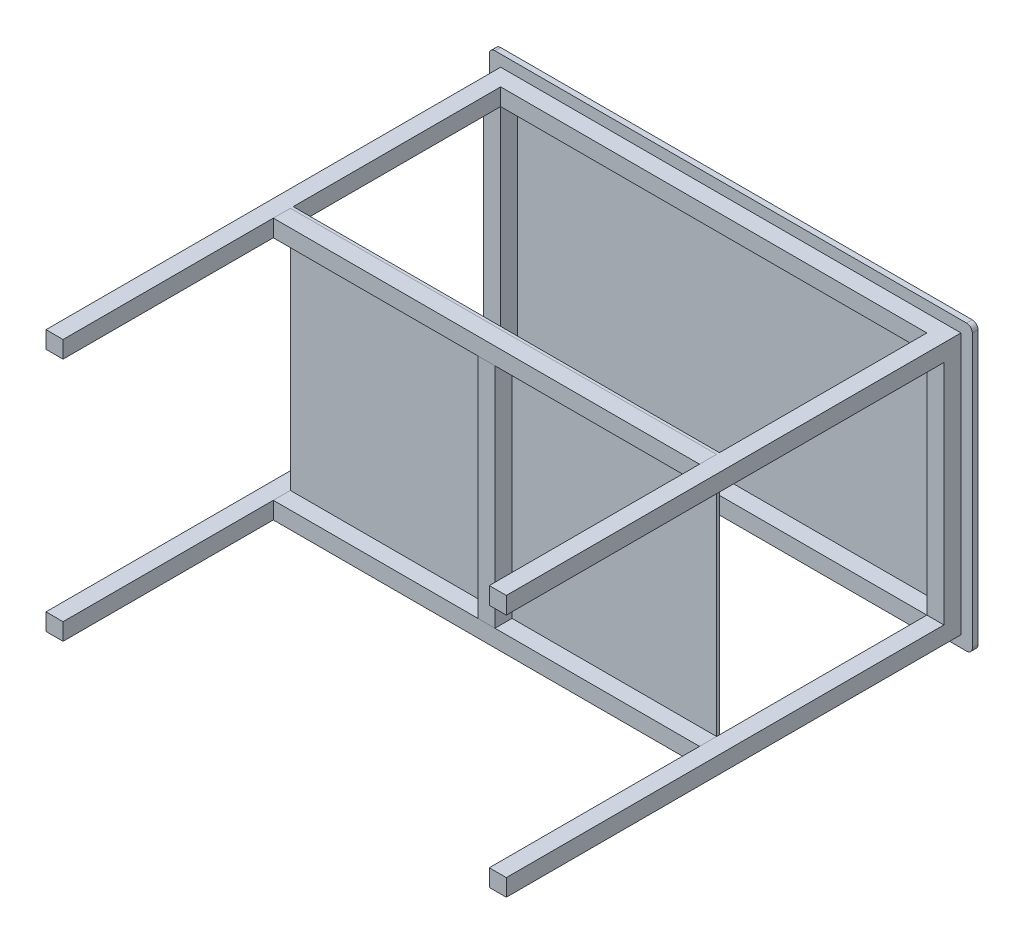
SolidWorks part; units mm, degrees
ref_plane "前视基准面" through (0, 0, 0) normal (0, 0, 1) x (1, 0, 0)
ref_plane "上视基准面" through (0, 0, 0) normal (0, 1, 0) x (1, 0, 0)
ref_plane "右视基准面" through (0, 0, 0) normal (1, 0, 0) x (0, 0, -1)
sketch "草图1" plane through (0, 0, 0) normal (0, 0, 1) x (1, 0, 0)
  line L1 (-425, 250) -> (425, 250)
  line L2 (-425, 250) -> (-425, -250)
  line L3 (-425, -250) -> (425, -250)
  line L4 (425, 250) -> (425, -250)
  line L5 (-425, 250) -> (425, -250) construction
  line L6 (-425, -250) -> (425, 250) construction
  point P0 (0, 0)
  dimension "D1" = 850
  dimension "D2" = 500
extrude "凸台-拉伸1" add sketch "草图1" along normal blind 10
sketch "草图2" plane through (0, 0, 10) normal (0, 0, 1) x (1, 0, 0)
  line L0 (425, 250) -> (-425, 250) construction
  line L1 (-405, 230) -> (405, 230)
  line L2 (-405, 230) -> (-405, -230)
  line L3 (-405, -230) -> (405, -230)
  line L4 (405, 230) -> (405, -230)
  line L5 (-405, 230) -> (405, -230) construction
  line L6 (-405, -230) -> (405, 230) construction
  line L7 (-425, 250) -> (-425, -250) construction
  line L8 (-375, 200) -> (-375, -200)
  line L9 (-375, -200) -> (375, -200)
  line L10 (375, 200) -> (375, -200)
  line L11 (-375, 200) -> (375, 200)
  point P0 (0, 0)
  dimension "D1" = 20
  dimension "D2" = 20
  dimension "D3" = 30
extrude "凸台-拉伸2" add sketch "草图2" along normal blind 30 separate body
sketch "草图3" plane through (0, 0, 40) normal (0, 0, 1) x (1, 0, 0)
  line L1 (-405, 230) -> (-375, 230)
  line L2 (-405, 230) -> (-405, 200)
  line L3 (-405, 200) -> (-375, 200)
  line L4 (-375, 230) -> (-375, 200)
  line L5 (375, -200) -> (405, -200)
  line L6 (375, -200) -> (375, -230)
  line L7 (375, -230) -> (405, -230)
  line L8 (405, -200) -> (405, -230)
  line L9 (405, 230) -> (375, 230)
  line L10 (405, 230) -> (405, 200)
  line L11 (405, 200) -> (375, 200)
  line L12 (375, 230) -> (375, 200)
  line L13 (-375, -200) -> (-405, -200)
  line L14 (-375, -200) -> (-375, -230)
  line L15 (-375, -230) -> (-405, -230)
  line L16 (-405, -200) -> (-405, -230)
extrude "凸台-拉伸3" add sketch "草图3" along normal blind 770
sketch "草图4" plane through (0, 230, 0) normal (0, 1, 0) x (1, 0, 0)
  line L0 (-375, -810) -> (-375, -40) construction
  line L1 (-375, -405) -> (375, -405)
  line L2 (-375, -405) -> (-375, -410)
  line L3 (-375, -410) -> (375, -410)
  line L4 (375, -405) -> (375, -410)
  line L5 (375, -810) -> (375, -40) construction
  line L6 (-375, -810) -> (-405, -810) construction
  point P8 (-390, -810)
  dimension "D1" = 5
  dimension "D2" = 400
extrude "凸台-拉伸4" add sketch "草图4" against normal up to surface (460 mm away)
sketch "草图6" plane through (0, -230, 0) normal (0, -1, 0) x (1, 0, 0)
  line L0 (-375, 810) -> (-375, 410) construction
  line L1 (375, 410) -> (-375, 410)
  line L2 (375, 410) -> (375, 440)
  line L3 (375, 440) -> (-375, 440)
  line L4 (-375, 410) -> (-375, 440)
  dimension "D1" = 30
extrude "凸台-拉伸7" add sketch "草图6" against normal blind 30 separate body
sketch "草图7" plane through (0, 230, 0) normal (0, 1, 0) x (1, 0, 0)
  line L1 (-375, -410) -> (375, -410)
  line L2 (-375, -410) -> (-375, -440)
  line L3 (-375, -440) -> (375, -440)
  line L4 (375, -410) -> (375, -440)
extrude "凸台-拉伸8" add sketch "草图7" against normal blind 30 separate body
sketch "草图8" plane through (0, 0, 440) normal (0, 0, 1) x (1, 0, 0)
  line L0 (-375, 200) -> (375, 200) construction
  line L1 (-15, -200) -> (15, -200)
  line L2 (-15, -200) -> (-15, 200)
  line L3 (-15, 200) -> (15, 200)
  line L4 (15, -200) -> (15, 200)
  line L5 (-15, -200) -> (15, 200) construction
  line L6 (-15, 200) -> (15, -200) construction
  point P0 (0, 0)
  dimension "D1" = 30
extrude "凸台-拉伸9" add sketch "草图8" against normal blind 30 separate body
fillet "圆角1" radius 10 4 edges at (425, 250, 5) (425, -250, 5) (-425, -250, 5) (-425, 250, 5)
